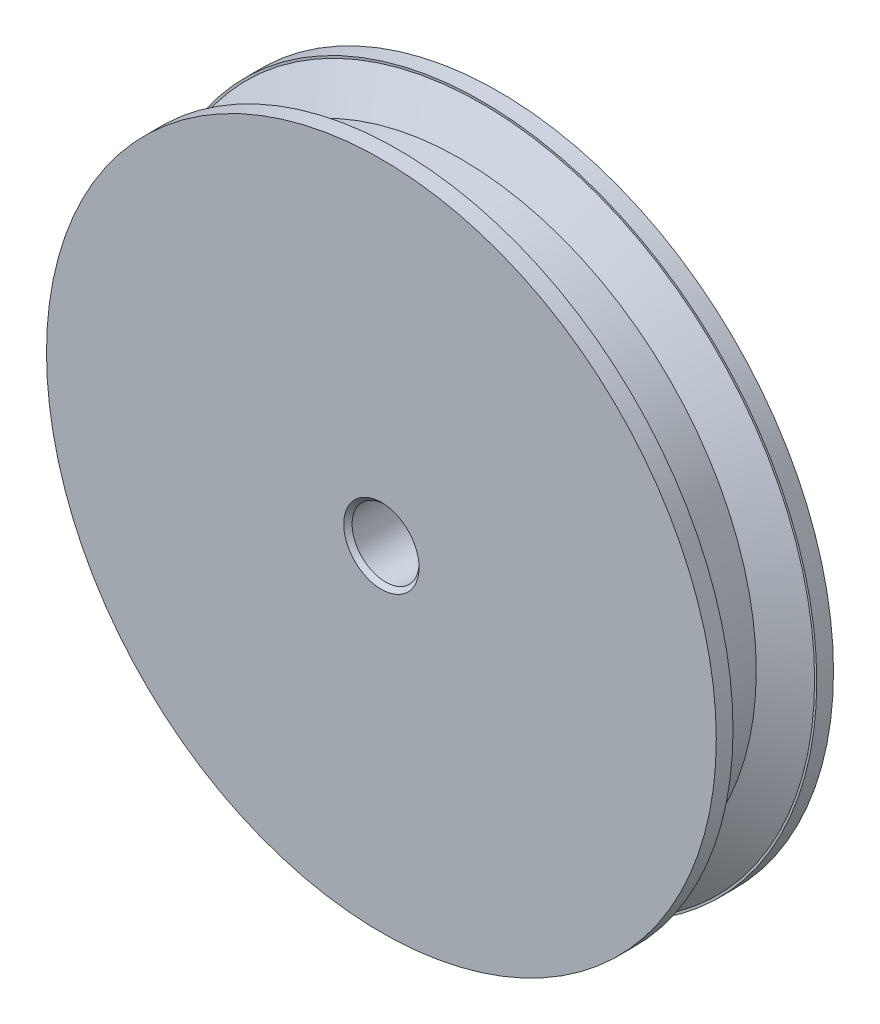
SolidWorks part; units mm, degrees
material "Plain carbon steel"
ref_plane "Front Plane" through (0, 0, 0) normal (0, 0, 1) x (1, 0, 0)
ref_plane "Top Plane" through (0, 0, 0) normal (0, 1, 0) x (1, 0, 0)
ref_plane "Right Plane" through (0, 0, 0) normal (1, 0, 0) x (0, 0, -1)
sketch "Sketch1" plane through (0, 0, 0) normal (0, 0, 1) x (1, 0, 0)
  circle A0 centre (0, 0) radius 40
  circle A1 centre (0, 0) radius 4
  dimension "D1" = 80
  dimension "D2" = 8
extrude "Boss-Extrude1" add sketch "Sketch1" along normal mid plane 14
sketch "Sketch2" plane through (0, 0, 0) normal (1, 0, 0) x (0, 0, -1)
  line L0 (0, 35.3253) -> (0, 40) construction
  line L1 (7, 40) -> (-7, 40) construction
  line L2 (-5, 39.7444) -> (-2.4486, 35.3253)
  line L3 (-2.4486, 35.3253) -> (2.4486, 35.3253)
  line L4 (2.4486, 35.3253) -> (5, 39.7444)
  line L5 (-5, 40) -> (5, 40)
  line L6 (7, 40) -> (-7, 40) construction
  line L12 (-7, 0) -> (7, 0) construction
  line L13 (-7, 40) -> (-7, -40) construction
  line L14 (7, -40) -> (7, 40) construction
  line L15 (-5, 40) -> (-5, 39.7444)
  line L16 (5, 40) -> (5, 39.7444)
  point P1 (-5.1476, 40)
  point P8 (5.1476, 40)
  point P30 (1, 25)
  dimension "D1" = 60
  dimension "D2" = 2
  dimension "D3" = 10
revolve "Cut-Revolve1" cut sketch "Sketch2" angle 360 about L12
chamfer "Chamfer1" distance 0.5 angle 45 2 edges at (4, 0, 7) (4, 0, -7)
